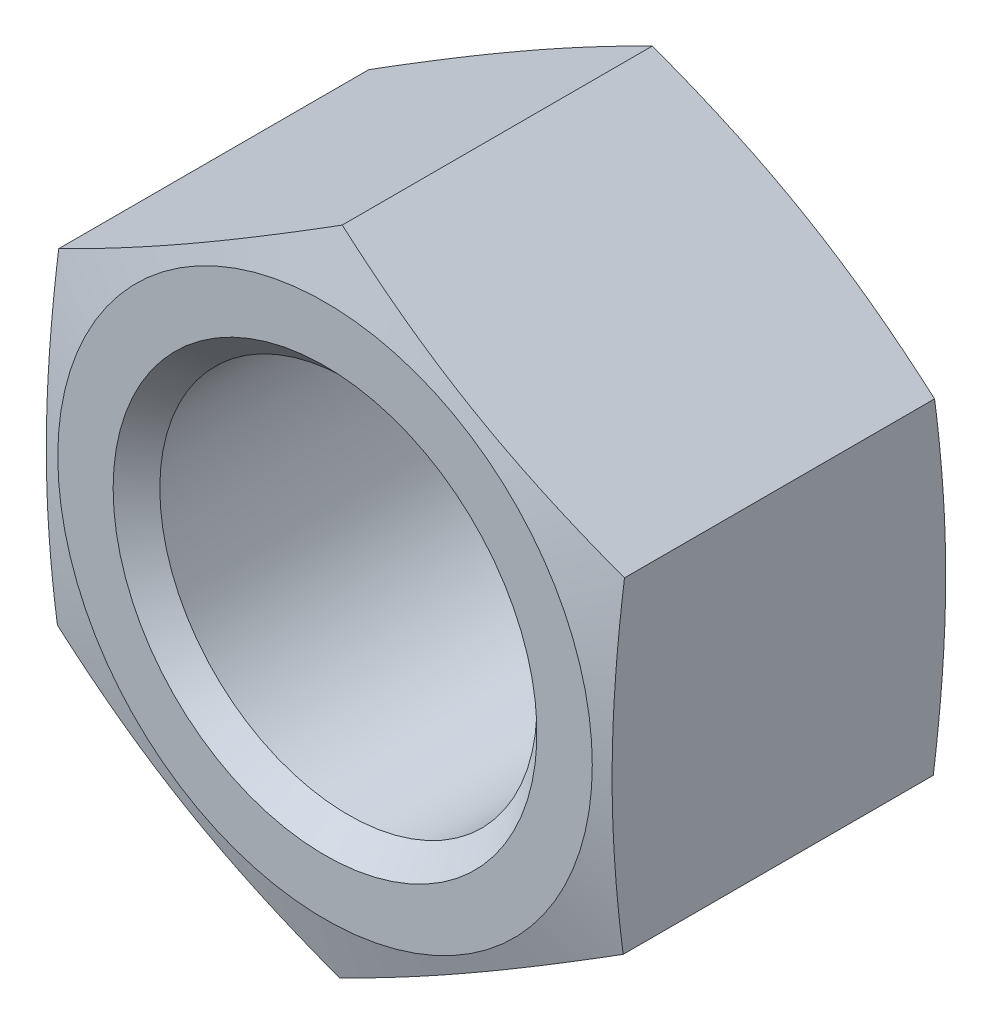
from build123d import *

# Parameters (mm, degrees)
SKETCH1_R          = 6.35
BASE_EXTRUDE_DEPTH = 11.38
SKETCH2_OUTSIDE_W  = 172.782
SKETCH2_OUTSIDE_H  = 175.686
SKETCH2_OUTSIDE_R  = 9.5
CUT_EXTRUDE1_DEPTH = 19.484149703
CUT_EXTRUDE1_DRAFT = -75
SKETCH3_OUTSIDE_W  = 172.782
SKETCH3_OUTSIDE_H  = 175.686
SKETCH3_OUTSIDE_R  = 9
CUT_EXTRUDE2_DEPTH = 19.484149703
CUT_EXTRUDE2_DRAFT = -75
CHAMFER1_SIZE      = 0.785714286


with BuildPart() as part:
    # Sketch1 → Base-Extrude (new body)
    with BuildSketch(Plane.XY):
        Polygon((0.043269974, 10.999914896), (-9.504570752, 5.537430344), (-9.547840726, -5.462484551), (-0.043269974, -10.999914896), (9.504570752, -5.537430344), (9.547840726, 5.462484551), align=None)
        Circle(SKETCH1_R, mode=Mode.SUBTRACT)
    extrude(amount=BASE_EXTRUDE_DEPTH)


with BuildPart() as cut_extrude1_tool:
    # Sketch2 outside → Cut-Extrude1 (with draft: the straight prism first)
    with BuildSketch(Plane(origin=(0, 0, 0), x_dir=(-1, 0, 0), z_dir=(0, 0, -1))):
        Rectangle(SKETCH2_OUTSIDE_W, SKETCH2_OUTSIDE_H)
        Circle(SKETCH2_OUTSIDE_R, mode=Mode.SUBTRACT)
    extrude(amount=-CUT_EXTRUDE1_DEPTH)
    # Cut-Extrude1: the draft: its side faces are tilted about the plane it starts from
    cut_extrude1_sides = [cut_extrude1_tool.faces().sort_by_distance(p)[0] for p in [
        (0, -87.843, 9.742074851),
        (-86.391, 0, 9.742074851),
        (0, 87.843, 9.742074851),
        (86.391, 0, 9.742074851),
        (9.5, 0, 9.742074851),
    ]]
    draft(cut_extrude1_sides, Plane(origin=(0, 0, 0), x_dir=(-1, 0, 0), z_dir=(0, 0, -1)), CUT_EXTRUDE1_DRAFT)


with BuildPart() as part_1:
    add(part.part)

    # Cut-Extrude1: cut by cut_extrude1_tool
    add(cut_extrude1_tool.part, mode=Mode.SUBTRACT)


with BuildPart() as cut_extrude2_tool:
    # Sketch3 outside → Cut-Extrude2 (with draft: the straight prism first)
    with BuildSketch(Plane.XY.offset(11.38)):
        Rectangle(SKETCH3_OUTSIDE_W, SKETCH3_OUTSIDE_H)
        Circle(SKETCH3_OUTSIDE_R, mode=Mode.SUBTRACT)
    extrude(amount=-CUT_EXTRUDE2_DEPTH)
    # Cut-Extrude2: the draft: its side faces are tilted about the plane it starts from
    cut_extrude2_sides = [cut_extrude2_tool.faces().sort_by_distance(p)[0] for p in [
        (0, -87.843, 1.637925149),
        (86.391, 0, 1.637925149),
        (0, 87.843, 1.637925149),
        (-86.391, 0, 1.637925149),
        (-9, 0, 1.637925149),
    ]]
    draft(cut_extrude2_sides, Plane.XY.offset(11.38), CUT_EXTRUDE2_DRAFT)


with BuildPart() as part_2:
    add(part_1.part)

    # Cut-Extrude2: cut by cut_extrude2_tool
    add(cut_extrude2_tool.part, mode=Mode.SUBTRACT)

    # Chamfer1
    chamfer1_edges = [part_2.edges().sort_by_distance(p)[0] for p in [
        (-6.35, 0, 0),
        (-6.35, 0, 11.38),
    ]]
    chamfer(chamfer1_edges, length=CHAMFER1_SIZE)


solid = part_2.part
